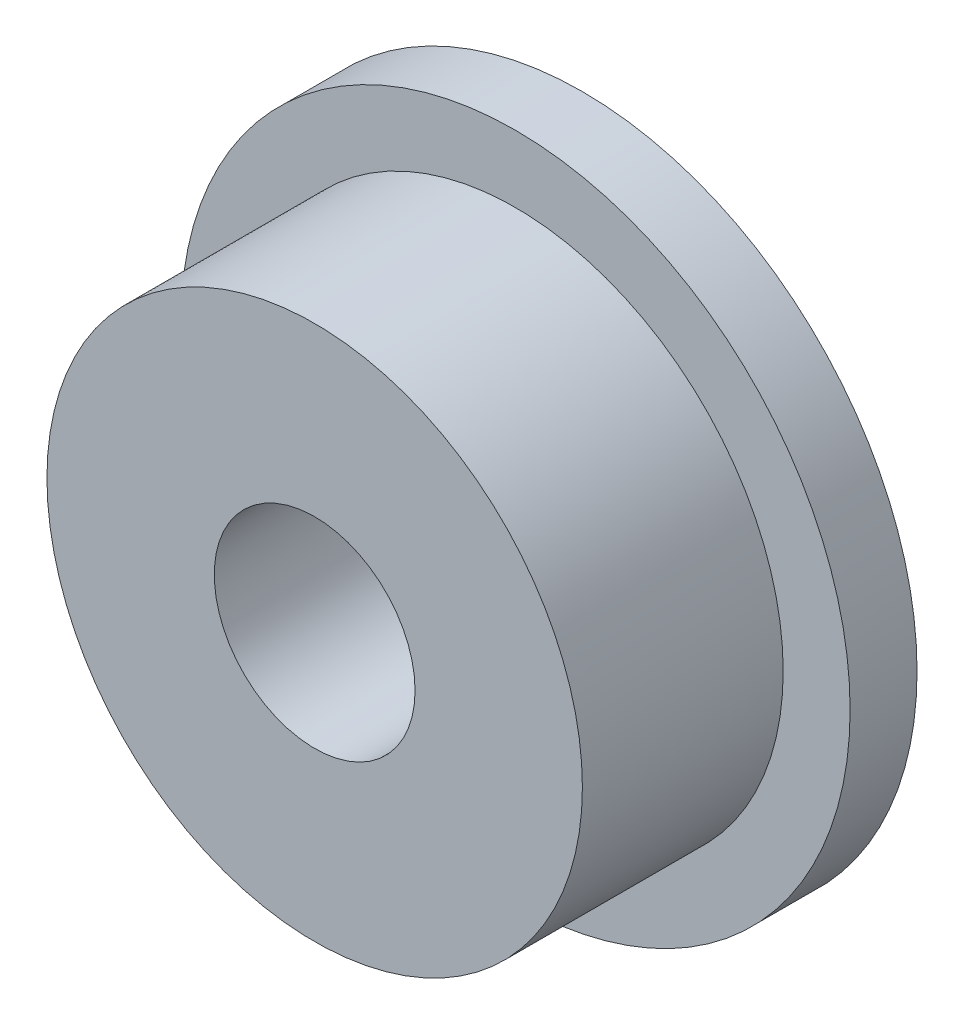
SolidWorks part; units mm, degrees
ref_plane "Front Plane" through (0, 0, 0) normal (0, 0, 1) x (1, 0, 0)
ref_plane "Top Plane" through (0, 0, 0) normal (0, 1, 0) x (1, 0, 0)
ref_plane "Right Plane" through (0, 0, 0) normal (1, 0, 0) x (0, 0, -1)
other "Configuration Table"
sketch "Sketch1" plane through (0, 0, 0) normal (0, 0, 1) x (1, 0, 0)
  circle A0 centre (0, 0) radius 5
  dimension "D1" = 10
extrude "Boss-Extrude1" add sketch "Sketch1" along normal blind 4
sketch "Sketch2" plane through (0, 0, 4) normal (0, 0, 1) x (1, 0, 0)
  circle A0 centre (0, 0) radius 4
  circle A1 centre (0, 0) radius 5
  circle A2 centre (0, 0) radius 5
  dimension "D2" = 8
  dimension "D1" = 0
extrude "Cut-Extrude1" cut sketch "Sketch2" against normal blind 3
sketch "Sketch3" plane through (0, 0, 4) normal (0, 0, 1) x (1, 0, 0)
  circle A0 centre (0, 0) radius 1.5
  dimension "D1" = 3
extrude "Cut-Extrude2" cut sketch "Sketch3" against normal through all and the other way through all
